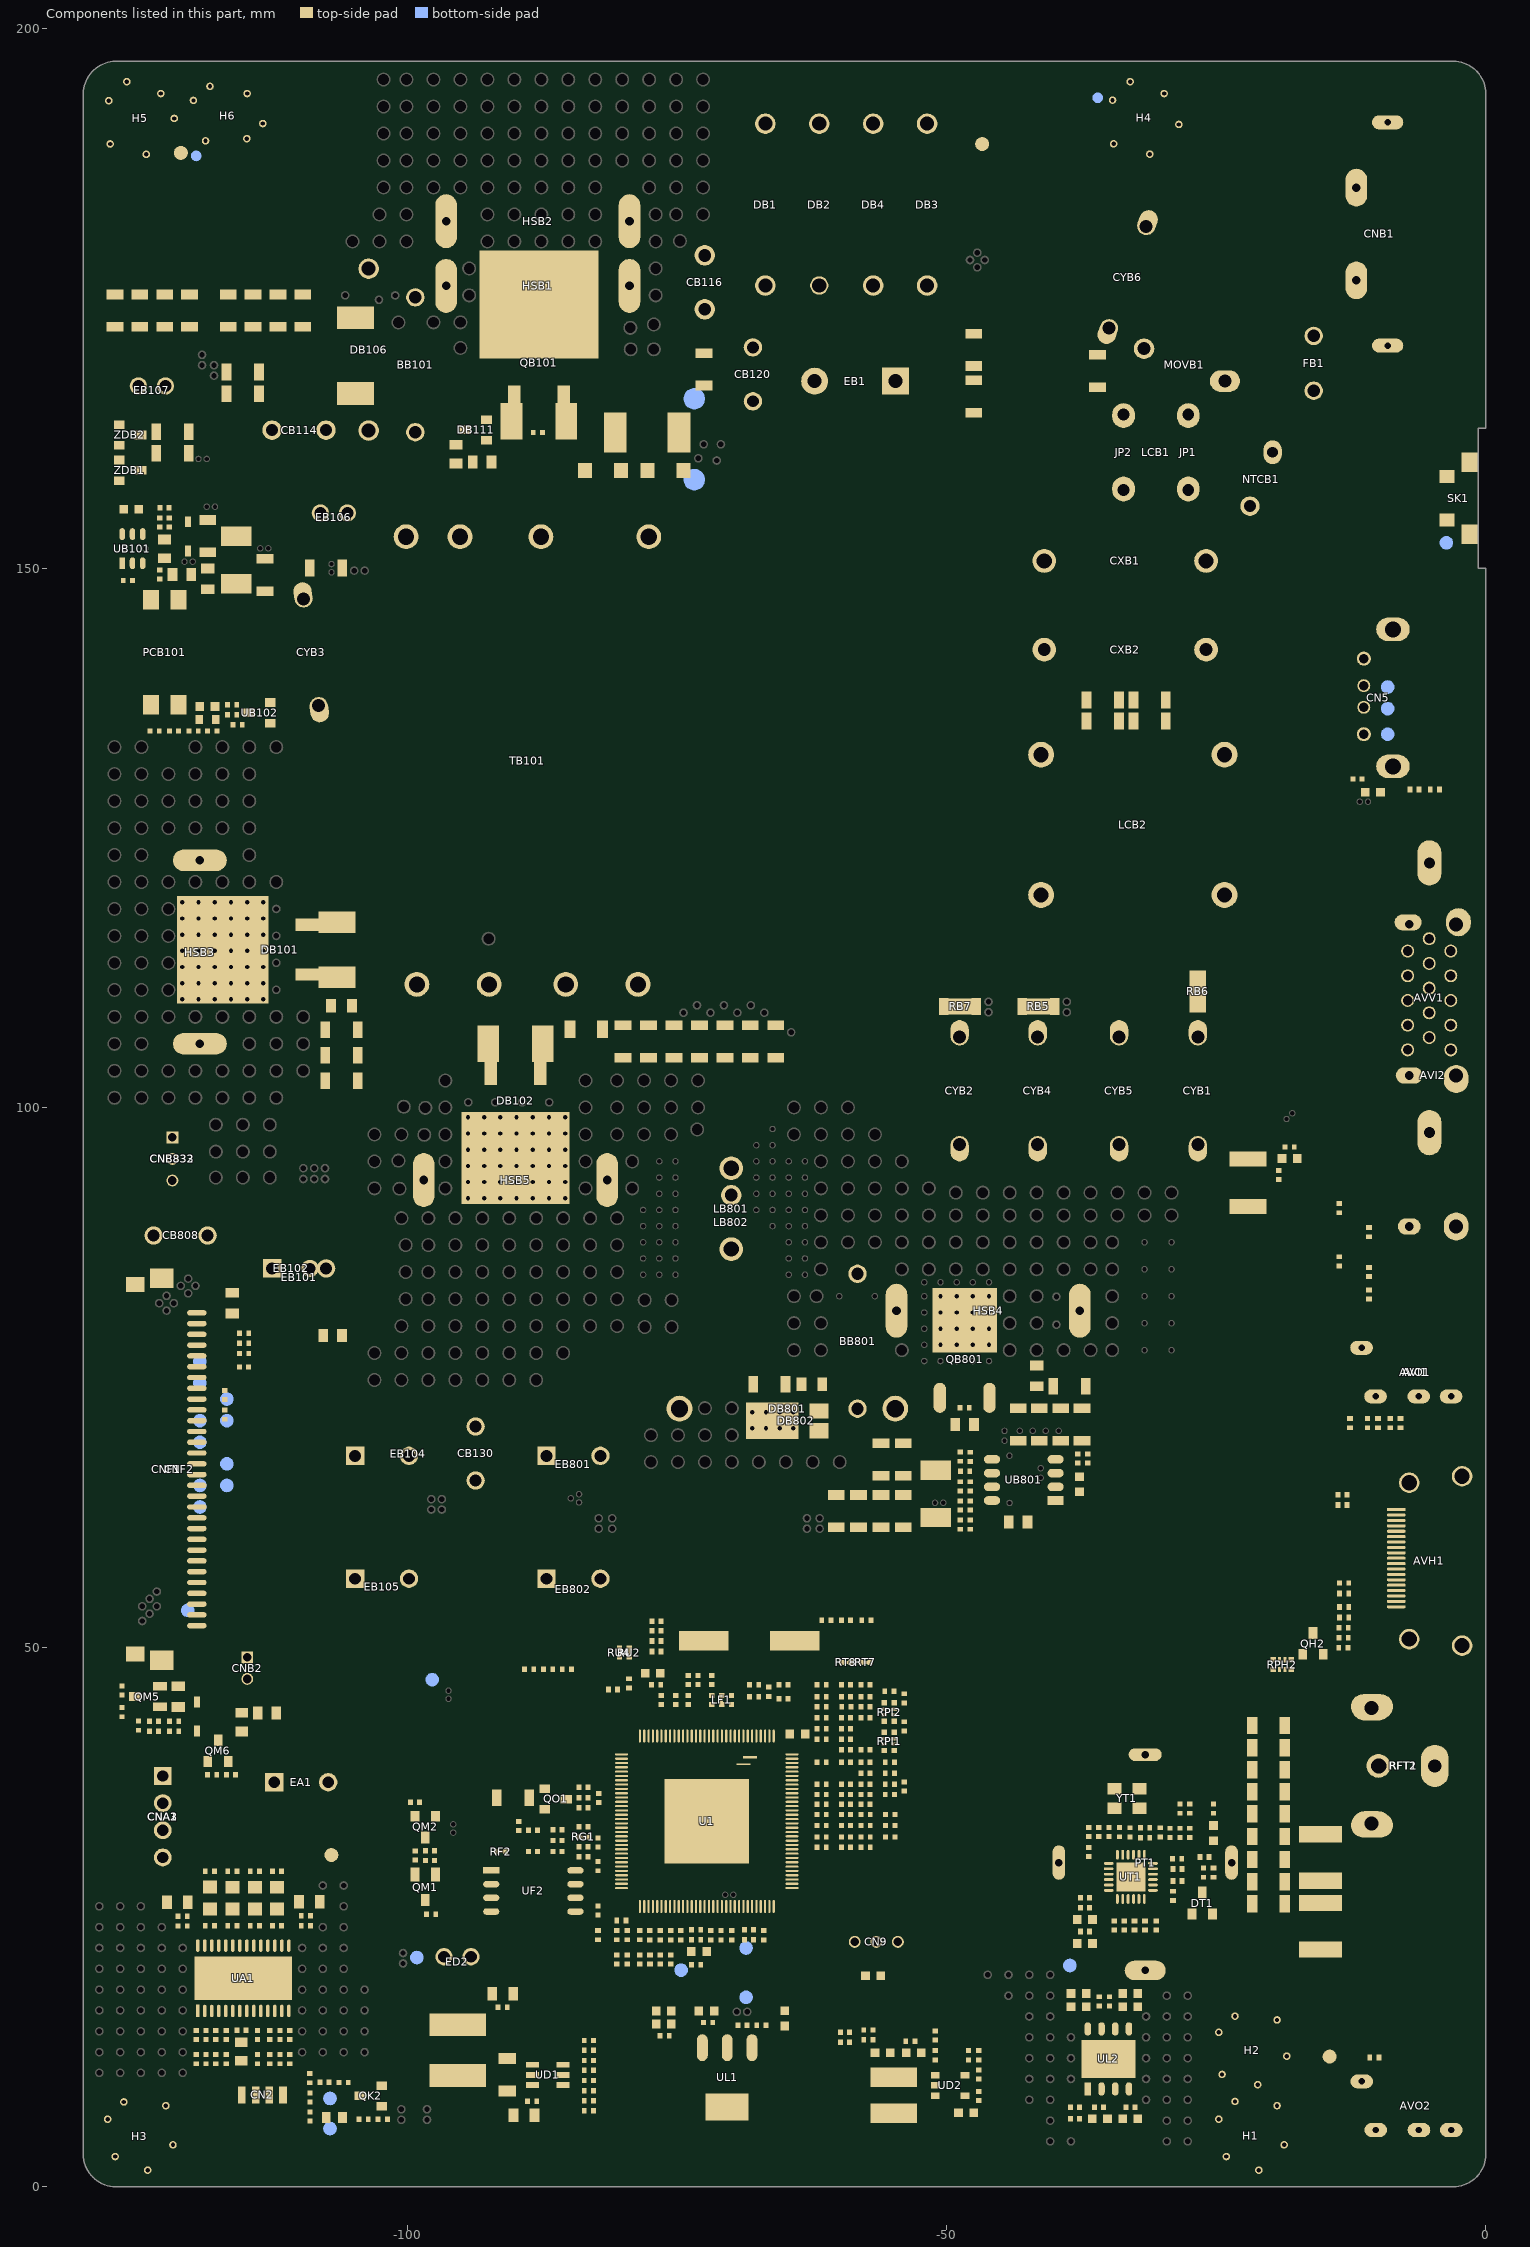
[diagram p0: the components of this part, seen from the top]
# Altium PCB MISC84438.PcbDoc (part 15 of 15)
Units mm, origin at the board's own origin, x right, y up, seen from the top; angles counter-clockwise.
Board outline 130 x 197 mm, 2 copper layers (TopLayer, BottomLayer), stack 1.571 mm thick; 574 components, 314 nets, 2636 pads, 811 vias.

## Silkscreen, mask and mechanical layers (free items; w line width, h text height) (continued)
BottomOverlay:
  circle w0.102: c-24.787,136.502 r0.051
  circle w0.15: c-24.787,135.35 r0.051
  circle w0.102: c-24.787,138.885 r0.051
  circle w0.15: c-24.787,137.733 r0.051
  circle w0.15: c-12.084,167.357 r0.051
  circle w0.102: c-12.084,168.509 r0.051
  circle w0.15: c-41.932,137.633 r0.051
  circle w0.102: c-41.932,138.785 r0.051
  circle w0.15: c-41.932,135.15 r0.051
  circle w0.102: c-41.932,136.302 r0.051
  rectangle: 172.367,19.026 175.674,21.026
  lines w0.127: -123.698,39.243 -127.762,39.243 -127.762,29.337 -123.571,29.337 ; -123.123,92.328 -124.837,92.328 -124.837,98.171 -123.055,98.171 ; -59.621,21.62 -59.621,18.191 -53.398,18.191 -53.398,21.613 ; -41.97,136.302 -41.932,135.502 -41.893,136.302 ; -41.97,138.785 -41.932,137.985 -41.893,138.785 ; -24.825,136.502 -24.787,135.702 -24.748,136.502 ; -24.825,138.885 -24.787,138.085 -24.748,138.885 ; -12.122,168.509 -12.084,167.709 -12.046,168.509 ; 186.36,19.026 186.36,21.026 ; -71.247,91.989 ccw(c-69.977,91.989) -69.977,90.719 -69.945,90.719 -69.926,90.719 ccw(c-69.926,91.989) -68.656,91.989 -68.656,94.513 ccw(c-69.85,94.513) -69.85,95.707 -69.926,95.707 -69.977,95.707 ccw(c-69.977,94.437) -71.247,94.437 -71.247,92.456 -71.247,91.989 ; -51.658,20.062 -51.658,31.562 -40.658,31.562 -40.658,20.062 -51.658,20.062 ; -43.19,134.859 -40.59,134.859 -41.94,136.809 -43.19,134.859 ; -43.19,137.342 -40.59,137.342 -41.94,139.292 -43.19,137.342 ; -33.166,42.659 -22.166,42.659 -22.166,54.159 -33.166,54.159 -33.166,42.659 ; -26.045,135.059 -24.795,137.009 -23.445,135.059 -26.045,135.059 ; -26.045,137.442 -24.795,139.392 -23.445,137.442 -26.045,137.442 ; -24.466,82.659 -24.466,94.159 -13.466,94.159 -13.466,82.659 -24.466,82.659 ; -13.342,167.066 -10.742,167.066 -12.092,169.016 -13.342,167.066 ; -13.177,52.133 -13.177,63.633 -2.177,63.633 -2.177,52.133 -13.177,52.133 ; 172.367,19.026 190.96,19.026 190.96,21.026 172.367,21.026 172.367,19.026
  lines w0.5: -43.1,33.038 -42.1,32.038 ; -42.1,35.438 -42.1,32.038 ; -41.1,33.038 -42.1,32.038 ; -24.608,55.797 -23.608,54.797 ; -23.608,58.197 -23.608,54.797 ; -22.608,55.797 -23.608,54.797 ; -15.908,95.797 -14.908,94.797 ; -14.908,98.197 -14.908,94.797 ; -13.908,95.797 -14.908,94.797 ; -5.405,65.271 -4.405,64.271 ; -4.405,67.671 -4.405,64.271 ; -3.405,65.271 -4.405,64.271 ; -129.481,139.692 -129.481,144.692 -96.952,144.692 -96.952,139.692 -129.481,139.692 ; -129.478,179.417 -110.92,179.417 -105.566,184.771 -105.566,196.478 -110.566,196.478 -110.566,186.792 -112.94,184.417 -129.478,184.417 -129.478,179.417 ; -80.629,124.507 -55.222,99.1 -22.029,99.1 -15.9,105.229 -15.9,143.18 -8.852,150.228 -8.852,160.731 -7.125,162.458 -1.219,162.458 -1.219,167.458 -9.196,167.458 -13.852,162.802 -13.852,152.299 -20.9,145.251 -20.9,107.3 -24.1,104.1 -53.151,104.1 -73.558,124.507 -80.629,124.507 ; -43.79,184.547 -43.79,196.481 -38.79,196.481 -38.79,186.618 -32.072,179.9 -29.771,179.9 -24.257,185.414 -24.257,196.481 -19.257,196.481 -19.257,183.343 -24.908,177.692 -27.7,174.9 -34.143,174.9 -43.79,184.547
  text "AC IN" at -16.637,179.578 h1.52 r270
  text "FB1" at -11.6,165.8 h1.27
  text "KEY" at -4.089,155.296 h1.52 r270
  text "USB IN" at -2.565,134.391 h1.52 r270
  text "VGA IN" at -1.665,108.699 h1.52 r270
  text "+" at -124.608,96.825 h2 r270
  text "NC" at -124.43,94.577 h1.3 r270
  text "AV2 IN" at -2.769,93.574 h1.52 r270
  text "-" at -124.684,92.888 h3 r270
  text "AV OUT(mini)" at -0.94,78.143 h1.52
  text "AV1 IN(mini)" at -0.94,76.683 h1.52
  text "XXXXXXXXXXXXXXX" at -53.581,58.293 h3.05
  text "XXXXXX" at -53.581,55.893 h3.05
  text "V3 2018.12.08" at -53.581,53.467 h3.05
  text "HDMI(ARC)(UART) IN" at -1.626,51.257 h1.52 r270
  text "RF IN" at -3.34,35.001 h1.52
  text ".GBO" at 186.988,19.611 h1.52
  text "BottomOverlay" at 176.277,19.586 h1.52
  text "GND" at -58.933,18.598 h1.27 r270
  text "RXD" at -56.921,18.593 h1.27 r270
  text "TXD" at -54.849,18.593 h1.27 r270
  text "EXT-IR" at -2.984,8.179 h1.52
  text "JX Label" at -58.6,5 h2.03
TopPaste:
  rectangle: 172.367,36.639 175.674,38.639
  lines w0.127: 186.36,36.639 186.36,38.639 ; 172.367,36.639 172.367,38.639 190.96,38.639 190.96,36.639 172.367,36.639
  text "TopPaste" at 176.569,37.178 h1.52
  text ".GTP" at 186.972,37.124 h1.52
BottomPaste:
  rectangle: 172.367,16.635 175.674,18.635
  lines w0.127: 186.36,16.635 186.36,18.635 ; 172.367,16.635 172.367,18.635 190.96,18.635 190.96,16.635 172.367,16.635
  text "BottomPaste" at 176.248,17.219 h1.52
  text ".GBP" at 186.995,17.089 h1.52
TopSolder:
  rectangle: 172.367,31.814 175.674,33.814
  lines w0.127: 186.36,31.814 186.36,33.814 ; 172.367,31.814 172.367,33.814 190.96,33.814 190.96,31.814 172.367,31.814
  text "TopSolder" at 176.582,32.325 h1.52
  text ".GTS" at 186.972,32.283 h1.52
BottomSolder:
  drawing of 44 lines, arcs and shapes, not listed
  text "BottomSolder" at 176.248,21.953 h1.52
  text ".GBS" at 186.971,21.931 h1.52
3D和装配:
  text "2L,2,130.00×197.00mm,FR4(TG130-CTI175),1OZ,Green,OSP,1.6mm,4,48,90.4%,2484,0.4mm" at 176.641,147.845 h1.52
自动测试:
  circle w0.152: c-112.42,62.323 r5
  circle w0.152: c-112.391,62.323 r6
  circle w0.152: c-40.011,179.938 r7
  circle w0.152: c-40.068,179.938 r5
  circle w0.152: c-40.039,179.938 r6
  circle w0.152: c-109.486,186.059 r5
  circle w0.152: c-109.458,186.059 r6
  circle w0.152: c-9.766,152.404 r5
  circle w0.152: c-15.735,122.991 r5
  circle w0.152: c-15.706,122.991 r6
  circle w0.152: c-45.678,45.953 r6
  circle w0.152: c-45.707,45.953 r5
  circle w0.152: c-45.649,45.953 r7
  circle w0.152: c-103.898,16.476 r5
  circle w0.152: c-48.171,30.027 r5
  circle w0.152: c-96.745,44.035 r6
  circle w0.152: c-96.774,44.035 r5
  circle w0.152: c-96.716,44.035 r7
顶层限制:
  drawing of 5135 lines, arcs and shapes, not listed
  text "虚线标注为蹇ㄗ畲蟪叽?" at -236.247,196.512 h3.6
  text "Top and bottom layers: no-component areas, routing allowed" at 1.712,193.636 h2
  text "Connector position is" at -91.044,151.345 h4
  text "Layout" at -62.44,151.345 h4
  text "Process" at -46.18,151.345 h4
  text "may still be adjusted" at -91.602,143.963 h4
  text "LED DRIVER" at -119.243,132.286 h3.6
  text "Note: connector compatibility here requires pad adjustment" at -51.823,112.584 h2
  text "(参考XXXXXXXXXXXXXXX削焊盘)，" at -52.326,108.904 h2
  text "14" at 11.698,108.217 h2.5 r90
  text "屏线从逑伦撸跫兜撞?" at -122.034,107.038 h4
  text "Add drag solder on the left (wave direction to the right)," at -51.834,105.224 h2
  text "Confirm with NPI after completion" at -51.845,101.545 h2
  text "部分注意预留补婢嗬?" at -122.057,99.656 h4
  text "14" at 11.743,94.217 h2.5 r90
  text "UHD" at -126.977,86.3 h3
  text "10" at -118.51,71.758 h1.27 r270
  text "LVDS (may adjust left/right shift per layout" at -116.292,65.583 h3
  text "20" at -118.509,61.758 h1.27 r270
  text "situation)" at -116.292,60.06 h3
  text "30" at -118.511,51.769 h1.27 r270
  text "SPK" at -126.182,21.675 h3.6
  text "Top and bottom layers: no-component areas, routing allowed" at -10.184,-3.909 h2
底层限制:
  rectangle: -9,193.5 0,195
  lines w0.127: -125,182.5 cw(c-125,192) -125,201.5 ; -9,193.5 -9,195 ; -9,193.5 -9,195 ; -9,193.5 -9,195 ; -9,193.5 0,193.5 ; -9,193.5 -9,195 ; -9,193.5 0,193.5 ; -9,193.5 -9,195 ; -9,193.5 0,193.5 ; -9,193.5 -9,195 ; -9,195 0,195 ; -9,195 0,195 ; -9,195 0,195 ; 0,193.5 0,195 ; 0,193.5 0,195
附加说明:
  lines w0.127: 275.819,143.586 304.521,143.586 ; 275.819,146.312 304.521,146.312 ; 275.819,149.038 304.521,149.038 ; 275.819,151.765 304.521,151.765 ; 275.819,154.491 312.154,154.491 ; 283.452,140.86 283.452,157.217 ; 304.521,140.86 304.521,157.217 ; 275.819,140.86 275.819,157.217 312.154,157.217 312.154,140.86 275.819,140.86
  lines w2: -1.079,3.099 -1.079,132.461
  lines w2.1: -118.212,178.41 -118.085,178.283 -118.085,171.272 -116.84,170.028 -97.155,170.028 -91.135,164.008 -78.054,164.008 -75.387,166.675 -75.387,174.904 -73.33,176.962 -71.425,176.962
  lines w3: -128.422,7.582 -128.422,83.883
  text "Template date:" at 220.037,155.389 h1.52
  text "Version cycle number" at 276.374,155.359 h1.52
  text "PCB designer" at 290.484,155.346 h1.52
  text "Customer" at 307.324,155.359 h1.52
  text "2018.09.18" at 228.216,155.3 h1.52
  text "Panel utilisation:" at 220.024,152.925 h1.52
  text "8X%" at 228.216,152.823 h1.52
  text "(Fill in for non-TV division projects)" at 233.042,152.823 h1.52
  text "XXXXXX" at 276.869,152.641 h1.52
  text "LCF  MXZ" at 284.591,152.62 h1.52
  text "XXXXXX" at 276.769,149.941 h1.52
  text "DXQ" at 284.591,149.92 h1.52
  text "XXXXXX" at 276.769,147.325 h1.52
  text "MXZ" at 284.591,147.304 h1.52
  text "COMPANY_A" at 305.521,147.299 h1.52
  text "[X, X-compatible SMD pads: separate stencil openings]" at 191.704,87.586 h1.52
  text "The notes below must be copied to the TopOverlay layer; one or two notes may be used" at 209.559,77.195 h1.52
  text "Only one barcode position on board; the other barcode must be attached to a component" at 248.133,77.121 h1.52
  text "SMD parts within 3.5mm of PCB clamp edge; production needs special control" at 191.652,75.112 h1.52
  text "No barcode position on board; barcode must be attached to a component" at 248.133,75.109 h1.52
  text "Customer special requirements; special process requirements; leave blank if none" at 191.603,72.243 h1.52
  text "Height values and designators of SMD parts over 2mm on the solder side; leave blank if none" at 191.603,69.703 h1.52
  text "Easily damaged part designators; leave blank if none" at 191.558,65.99 h1.52
  text "New footprint designators; leave blank if none" at 191.618,60.731 h1.52
  text "X.XXXX.XXX Stencil Revision Explanation" at 168.088,-16.048 h1.52
  text "X.XXXX.XXX Testing jig Revision Explanation" at 168.075,-17.8 h1.52
  text "X.XXXX.XXX Wave-soldering jig Revision Explanation" at 168.063,-19.528 h1.52
DrillDrawing:
  text ".Legend" at 168.292,158.442 h1.52